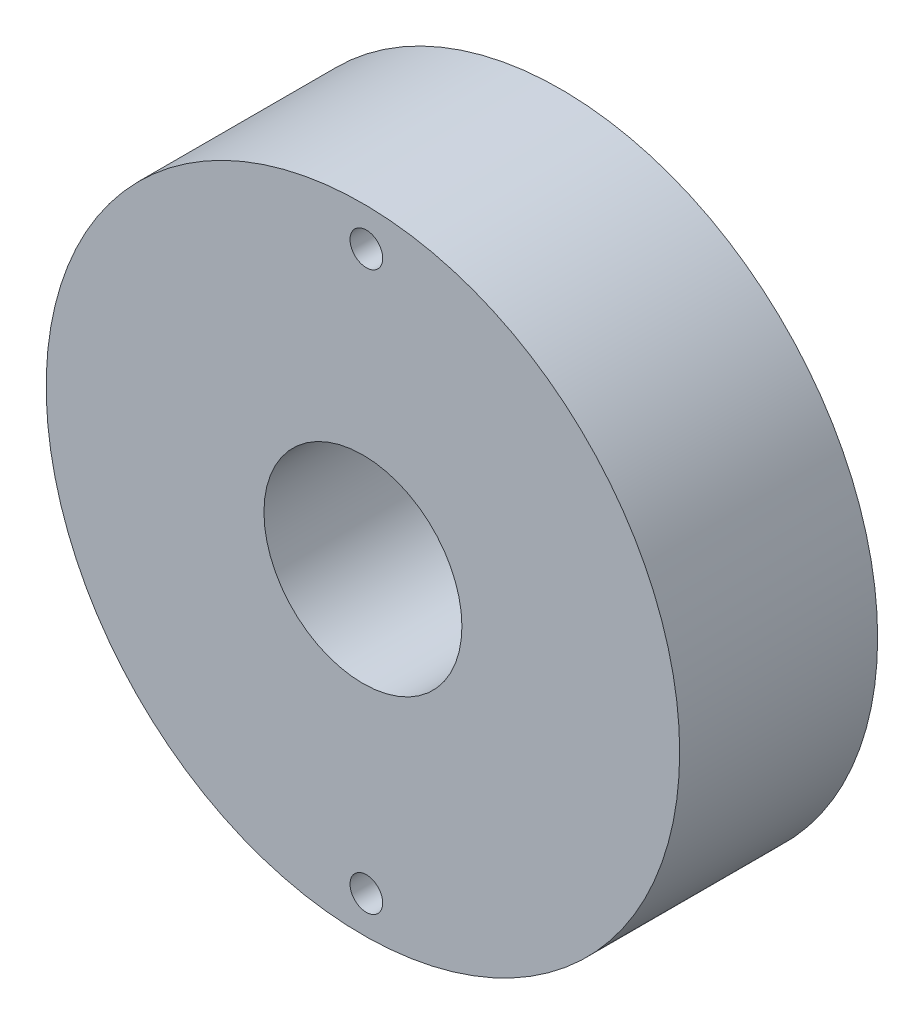
SolidWorks part; units mm, degrees
ref_plane "前视基准面" through (0, 0, 0) normal (0, 0, 1) x (1, 0, 0)
ref_plane "上视基准面" through (0, 0, 0) normal (0, 1, 0) x (1, 0, 0)
ref_plane "右视基准面" through (0, 0, 0) normal (1, 0, 0) x (0, 0, -1)
sketch "草图1" plane through (0, 0, 0) normal (0, 0, 1) x (1, 0, 0)
  circle A0 centre (-0.3472, 0) radius 10
  circle A1 centre (-0.3472, 0) radius 32
  dimension "D1" = 20
  dimension "D2" = 64
extrude "凸台-拉伸1" add sketch "草图1" along normal blind 20
hole_wizard "M4 螺纹孔3" positions "草图5" profile "草图6" tap size "M4" standard "GB"
sketch "草图5" plane through (0, 0, 0) normal (0, 0, -1) x (-1, 0, 0)
  line L0 (0, -35.4182) -> (0, 45.6703) construction
  point P0 (0, 28.2)
  point P2 (0, -28.2)
  dimension "D1" = 28.2
  dimension "D2" = 28.2
sketch "草图6" plane through (0, 28.2, 0) normal (1, 0, 0) x (0, 1, 0)
  line L0 (0, 0) -> (0, 33.0914)
  line L1 (0, 33.0914) -> (1.65, 32.1)
  line L2 (1.65, 32.1) -> (1.65, 0)
  line L5 (1.65, 0) -> (0, 0)
  line L10 (0, 33.0914) -> (-1.65, 32.1) construction
  line L11 (0, -6.35) -> (0, 107.95) construction
  dimension "螺纹孔钻头直径" = 3.3
  dimension "螺纹孔钻头深度" = 32.1
  dimension "导头角度" = 118
cosmetic thread "孔螺蚊线4"
cosmetic thread "孔螺蚊线5"
